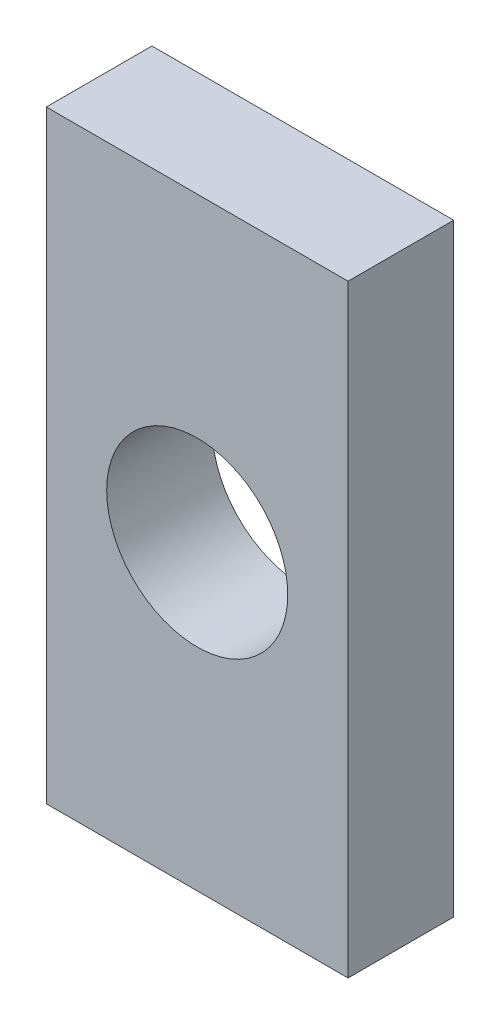
SolidWorks part; units mm, degrees
material "Plain carbon steel"
ref_plane "Front Plane" through (0, 0, 0) normal (0, 0, 1) x (1, 0, 0)
ref_plane "Top Plane" through (0, 0, 0) normal (0, 1, 0) x (1, 0, 0)
ref_plane "Right Plane" through (0, 0, 0) normal (1, 0, 0) x (0, 0, -1)
sketch "Sketch1" plane through (0, 0, 0) normal (0, 0, 1) x (1, 0, 0)
  line L0 (0, 0) -> (40, 0)
  line L1 (40, 0) -> (40, 80)
  line L2 (40, 80) -> (0, 80)
  line L3 (0, 80) -> (0, 0)
  circle A0 centre (20, 40) radius 12
  dimension "D3" = 24
  dimension "D1" = 40
  dimension "D2" = 80
  dimension "D4" = 40
  dimension "D5" = 20
extrude "Boss-Extrude1" add sketch "Sketch1" along normal blind 14
